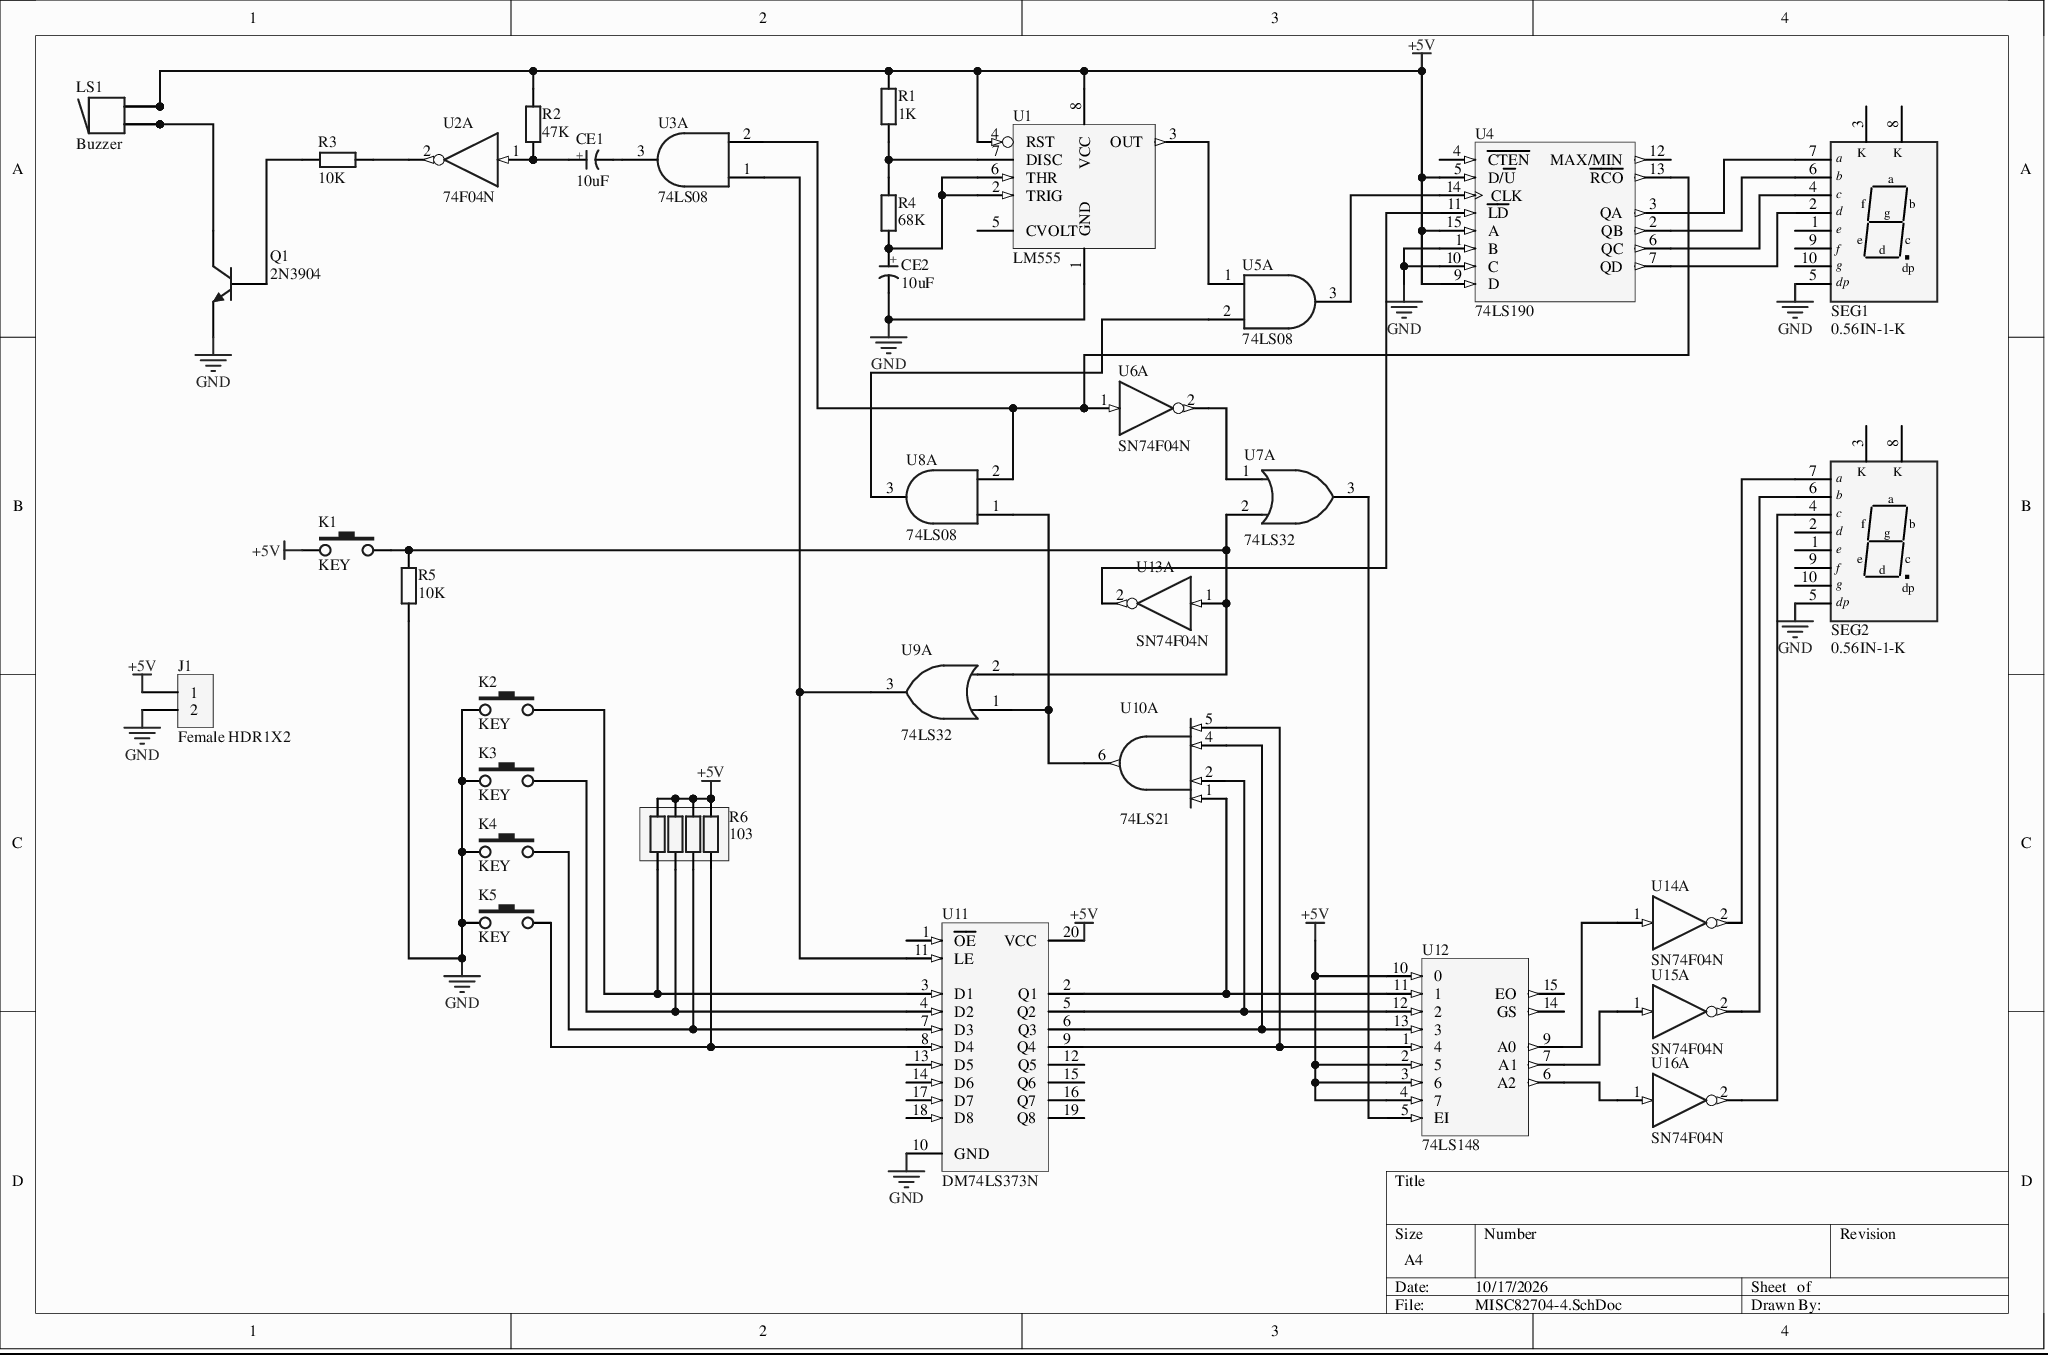
[diagram p0: MISC82704-4.SchDoc]
# Altium project MISC82704-7.PrjPcb
1 sheet, 34 parts. Net scope: global (net labels, ports and power ports of the same name join across sheets).
Board file: MISC82704.PcbDoc

## Sheet MISC82704-4.SchDoc
size A4

### Parts
CE1  10uF  [CAP 1.5*4*8]
CE2  10uF  [CAP 1.5*4*8]
J1  Female HDR1X2  [Fe-HDR1X2/2.54-S]
K1  KEY  [四脚轻触开关]
K2  KEY  [四脚轻触开关]
K3  KEY  [四脚轻触开关]
K4  KEY  [四脚轻触开关]
K5  KEY  [四脚轻触开关]
LS1  Buzzer  [ABSM-1574]
Q1  2N3904  [TO-92A]
R1  1K  [RS 1/4W]
R2  47K  [RS 1/4W]
R3  10K  [RS 1/4W]
R4  68K  [RS 1/4W]
R5  10K  [RS 1/4W]
R6  103  [RCA-8P4R-0603]
SEG1  0.56IN-1-K  [0.56IN-1P]
SEG2  0.56IN-1-K  [0.56IN-1P]
U1  LM555  [J08A]
U2  74F04N  [DIP14]  (part A of 6)
U3  74LS08  [DIP14]  (part A of 4)
U4  74LS190  [DIP16]
U5  74LS08  [DIP14]  (part A of 4)
U6  SN74F04N  [DIP14]  (part A of 6)
U7  74LS32  [DIP14]  (part A of 4)
U8  74LS08  [DIP14]  (part A of 4)
U9  74LS32  [DIP14]  (part A of 4)
U10  74LS21  [DIP14]  (part A of 2)
U11  DM74LS373N  [DIP20]
U12  74LS148  [DIP16]
U13  SN74F04N  [DIP14]  (part A of 6)
U14  SN74F04N  [DIP14]  (part A of 6)
U15  SN74F04N  [DIP14]  (part A of 6)
U16  SN74F04N  [DIP14]  (part A of 6)

### Nets
+5V: J1.1 K1.1 LS1.2 LS1.2A R1.2 R2.2 R6.5 R6.6 R6.7 R6.8 U1.4(RST) U1.8(VCC) U4.5(D/~{U}) U4.9(D) U4.15(A) U11.20(VCC) U12.2(5) U12.3(6) U12.4(7) U12.10(0)
GND: CE2.2(K) J1.2 K2.1 K3.1 K4.1 K5.1 Q1.1(E) R5.1 SEG1.5 SEG2.5 U1.1(GND) U2.7(GND) U4.1(B) U4.8(GND) U4.10(C) U6.7(GND) U10.7(GND) U11.10(GND) U12.8(GND) U13.7(GND) U14.7(GND) U15.7(GND) U16.7(GND)
VCC: U2.14(VCC) U4.16(VCC) U6.14(VCC) U10.14(VCC) U12.16(VCC) U13.14(VCC) U14.14(VCC) U15.14(VCC) U16.14(VCC)
NetCE1_1: CE1.1(A) R2.1 U2.1(A)
NetCE1_2: CE1.2(K) U3.3(Y)
NetCE2_1: CE2.1(A) R4.1 U1.2(TRIG) U1.6(THR)
NetK1_3: K1.3 R5.2 U7.2(B) U9.2(B) U13.1(A)
NetK2_3: K2.3 R6.1 U11.3(D1)
NetK3_3: K3.3 R6.2 U11.4(D2)
NetK4_3: K4.3 R6.3 U11.7(D3)
NetK5_3: K5.3 R6.4 U11.8(D4)
NetLS1_1: LS1.1 LS1.1A Q1.3(C)
NetQ1_2: Q1.2(B) R3.1
NetR1_1: R1.1 R4.2 U1.7(DISC)
NetR3_2: R3.2 U2.2(~{O})
NetSEG1_2: SEG1.2 U4.7(QD)
NetSEG1_4: SEG1.4 U4.6(QC)
NetSEG1_6: SEG1.6 U4.2(QB)
NetSEG1_7: SEG1.7 U4.3(QA)
NetSEG2_4: SEG2.4 U16.2(Y)
NetSEG2_6: SEG2.6 U15.2(Y)
NetSEG2_7: SEG2.7 U14.2(Y)
NetU1_3: U1.3(OUT) U5.1(A)
NetU3_1: U3.1(A) U9.3(Y) U11.11(LE)
NetU3_2: U3.2(B) U4.13(~{RCO}) U6.1(A) U8.2(B)
NetU4_11: U4.11(~{LD}) U13.2(Y)
NetU4_14: U4.14(CLK) U5.3(Y)
NetU5_2: U5.2(B) U8.3(Y)
NetU6_2: U6.2(Y) U7.1(A)
NetU7_3: U7.3(Y) U12.5(EI)
NetU8_1: U8.1(A) U9.1(A) U10.6(Y)
NetU10_1: U10.1(A) U11.2(Q1) U12.11(1)
NetU10_2: U10.2(B) U11.5(Q2) U12.12(2)
NetU10_4: U10.4(C) U11.6(Q3) U12.13(3)
NetU10_5: U10.5(D) U11.9(Q4) U12.1(4)
NetU12_6: U12.6(A2) U16.1(A)
NetU12_7: U12.7(A1) U15.1(A)
NetU12_9: U12.9(A0) U14.1(A)

Not connected (* = marked no-connect by the designer): SEG1 1 3(VCC) 8 9 10; SEG2 1 2 3(VCC) 8 9 10; U1 5(CVOLT); U3 7(GND) 14(VCC); U4 4(~{CTEN})* 12(MAX/MIN); U5 7(GND) 14(VCC); U7 7(GND) 14(VCC); U8 7(GND) 14(VCC); U9 7(GND) 14(VCC); U11 1(~{OE})* 12(Q5) 13(D5)* 14(D6)* 15(Q6) 16(Q7) 17(D7)* 18(D8)* 19(Q8); U12 14(GS) 15(EO)

### Library data of the parts
CE1 CE2 = CE: Through-hole electrolytic capacitor; BOM名称: Through-hole electrolytic capacitor
LS1 = Buzzer: Magnetic Transducer Buzzer; Published: 24-Mar-1999; LatestRevisionDate: 17-Dec-2003; LatestRevisionNote: Schematic revised, PCB Footprint replaced.; DatasheetVersion: 17-Dec-2003; PackageReference: ABSM-1574; PackageDescription: Magnetic Transducer Buzzer; ComponentLink1Description: Manufacturer Link; Publisher: Altium Limited
Q1 = 2N3904: NPN General Purpose Amplifier; Published: 8-Jun-2000; LatestRevisionDate: 15-Jan-2003; LatestRevisionNote: PCB Footprint 'BCY-W3/D4.7' replaced; DatasheetVersion: 1997; PackageVersion: Sep-1998; PackageReference: TO-92A; PackageDescription: TO, Flat Index; 3 In-Line, Axial Leads; Body Dia. 4.5mm; Leads 0.51 x 0.48 mm (max); ComponentLink1Description: Manufacturer Link; ComponentLink2Description: Datasheet; ComponentLink2URL: http://www.fairchildsemi.com/ds/2N%2F2N3904.pdf; Publisher: Altium Limited
R1-R5 = R-S: Color-band resistor; BOM名称: Color-band resistor
R6 = R-8P4R: SMD resistor network; BOM名称: SMD resistor network
SEG1 SEG2 = 0.56IN-1-K: 1-digit 0.56-inch common-cathode display
U1 = LM555J: Timer; Package Information: Latest Revision: 2000; Published: 15-Apr-2002; Datasheet: Latest Revision: May-1997; Package Reference: J08A; Publisher: Altium Limited
U2 = 74F04PC: Hex Inverter; Package Information: Latest Revision: 2000; Published: 15-Apr-2002; Datasheet: Latest Revision: Nov-1994; Package Reference: N14A; Publisher: Altium Limited
U3 U5 U8 = 74LS08: Quad 2-input AND gate
U4 = 74LS190: Synchronous 4-Bit Up/Down Decade Counter with Down/Up Mode Control
U6 U13-U16 = SN74F04N: Hex Inverter; Package Information: Latest Revision: Oct-1995; Published: 8-Jun-2000; Revision: 17-Jul-2002: Re-released for DXP Platform.; Datasheet: Latest Revision: Oct-1993; Package Reference: N014; Publisher: Altium Limited
U7 U9 = 74LS32: Quad 2-input OR gate
U10 = 74LS21: Dual 4-Input Positive-AND Gate
U11 = DM74LS373N: Tri-State Octal D-Type Transparent Latch and Edge-Triggered Flip-Flop; Package Information: Latest Revision: 2000; Note: Generic Sim model provided.; Code - JEDEC: MS-001-AD; Published: 15-Apr-2002; Datasheet: Latest Revision: May-1992; Package Reference: N20A; Publisher: Altium Limited
U12 = 74LS148: 8-Line to 3-Line Priority Encoder